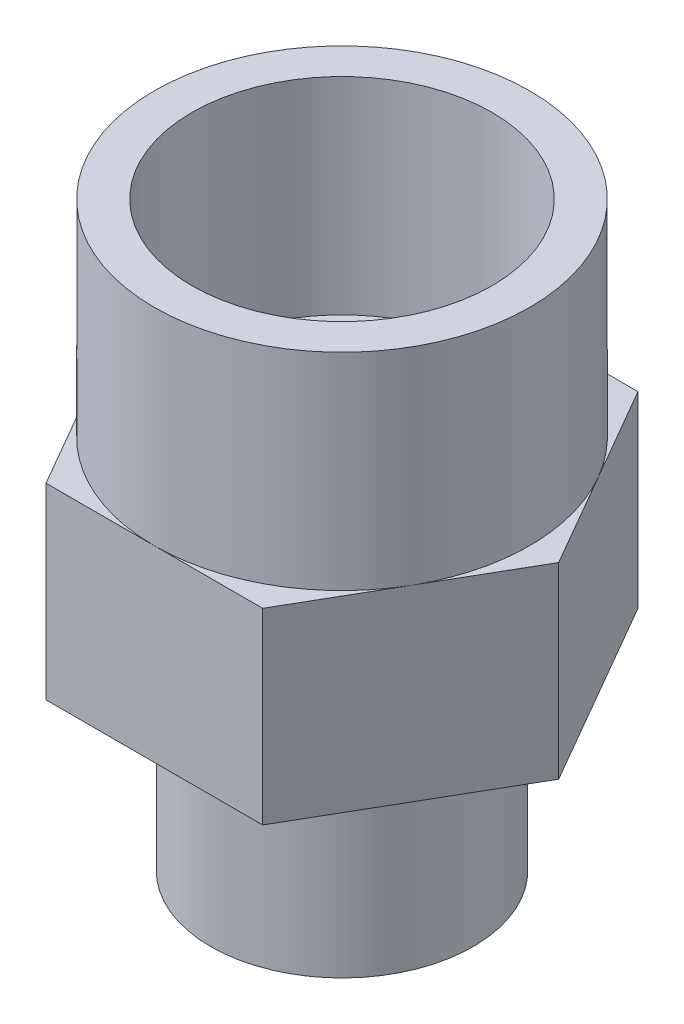
from build123d import *

# Parameters (mm, degrees)
SKETCH_1_R        = 10
SKETCH_1_R_2      = 8
EXTRUDE_1_DEPTH   = 11
SKETCH_2_R        = 5
EXTRUDE_1_2_DEPTH = 10
SKETCH_3_R        = 7
SKETCH_3_R_2      = 5
EXTRUDE_2_DEPTH   = 10


with BuildPart() as part:
    # 草图1 → Extrude 1 (new body)
    with BuildSketch(Plane(origin=(0, 0, 0), x_dir=(1, 0, 0), z_dir=(0, 1, 0))):
        Circle(SKETCH_1_R)
        Circle(SKETCH_1_R_2, mode=Mode.SUBTRACT)
    extrude(amount=EXTRUDE_1_DEPTH)

    # 草图2 → Extrude 1 2 (add)
    with BuildSketch(Plane.XZ):
        Polygon((11.547005384, 0), (5.773502692, 10), (-5.773502692, 10), (-11.547005384, 0), (-5.773502692, -10), (5.773502692, -10), align=None)
        with Locations(Location((0, 0, 0), (0, 0, 270))):
            Circle(SKETCH_2_R, mode=Mode.SUBTRACT)
    extrude(amount=EXTRUDE_1_2_DEPTH)

    # 草图3 → 拉伸-薄壁2 (add)
    with BuildSketch(Plane.XZ.offset(10)):
        Circle(SKETCH_3_R)
        Circle(SKETCH_3_R_2, mode=Mode.SUBTRACT)
    extrude(amount=EXTRUDE_2_DEPTH)


solid = part.part
